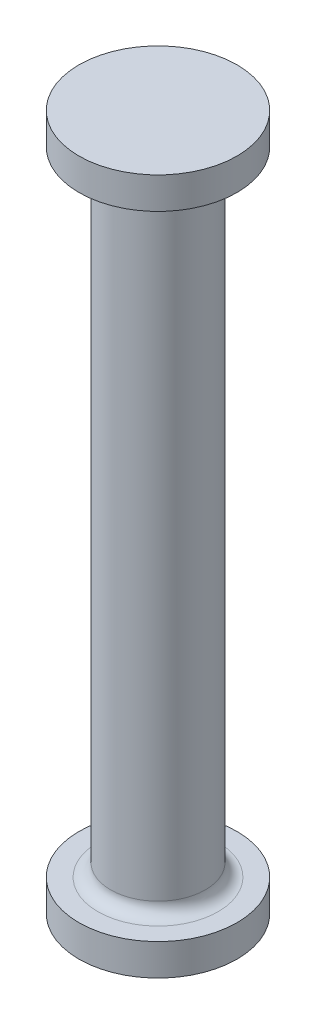
from build123d import *

# Parameters (mm, degrees)
FILLET_1_R = 2


with BuildPart() as part:
    # 草图1 → 旋转2 (revolve)
    with BuildSketch(Plane.XY, mode=Mode.PRIVATE) as revolve_2_sk:
        Polygon((0, -50), (0, 60), (12.5, 60), (12.5, 55), (7.5, 55), (7.5, -45), (12.5, -45), (12.5, -50), align=None)
    revolve(revolve_2_sk.sketch.rotate(Axis((0, -50, 0), (0, 1, 0)), 90), axis=Axis((0, -50, 0), (0, 1, 0)))

    # 圆角1
    fillet_1_edges = [part.edges().sort_by_distance(p)[0] for p in [
        (0, -45, 7.5),
        (0, 55, 7.5),
    ]]
    fillet(fillet_1_edges, radius=FILLET_1_R)


solid = part.part
